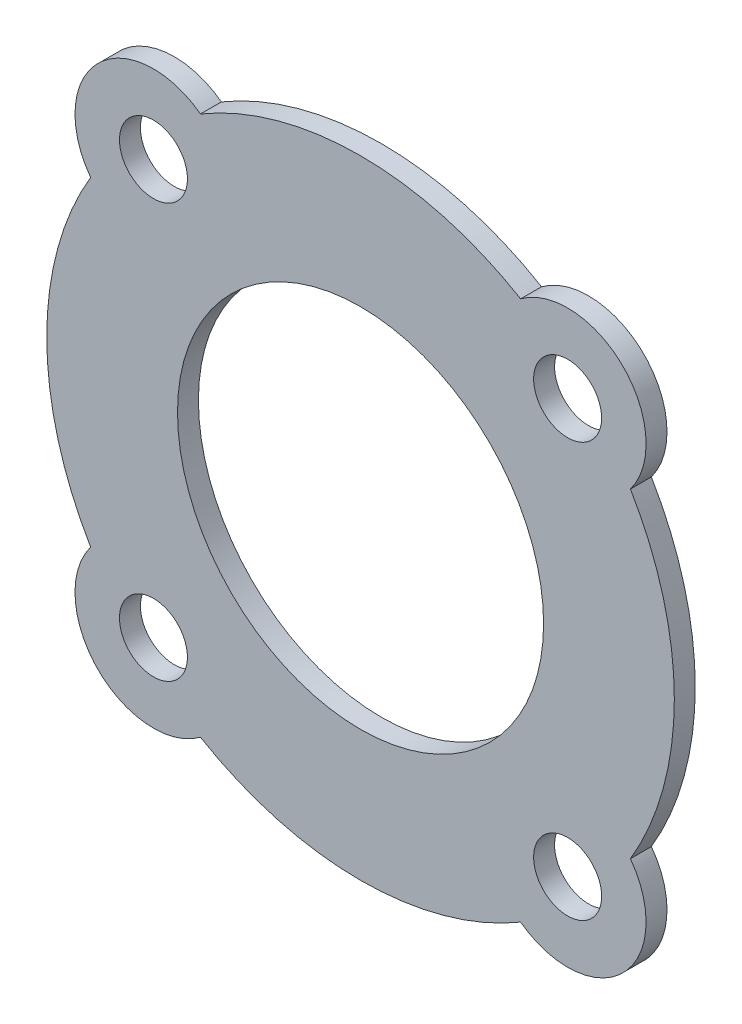
SolidWorks part; units mm, degrees
ref_plane "Front Plane" through (0, 0, 0) normal (0, 0, 1) x (1, 0, 0)
ref_plane "Top Plane" through (0, 0, 0) normal (0, 1, 0) x (1, 0, 0)
ref_plane "Right Plane" through (0, 0, 0) normal (1, 0, 0) x (0, 0, -1)
sketch "Sketch1" plane through (0, 0, 0) normal (0, 0, 1) x (1, 0, 0)
  line L0 (0, 0) -> (0, 56)
  line L1 (39.598, 39.598) -> (0, 0) construction
  circle A0 centre (0, 0) radius 35
  circle A1 centre (0, 0) radius 56 construction
  arc A2 (30.6082, 51.6056) -> (-30.6082, 51.6056) centre (0, 0) ccw
  circle A3 centre (39.598, 39.598) radius 6.5
  arc A4 (51.6056, 30.6082) -> (30.6082, 51.6056) centre (39.598, 39.598) ccw
  arc A5 (30.6082, -51.6056) -> (51.6056, -30.6082) centre (39.598, -39.598) ccw
  circle A6 centre (39.598, -39.598) radius 6.5
  arc A7 (-51.6056, -30.6082) -> (-30.6082, -51.6056) centre (-39.598, -39.598) ccw
  circle A8 centre (-39.598, -39.598) radius 6.5
  arc A9 (-30.6082, 51.6056) -> (-51.6056, 30.6082) centre (-39.598, 39.598) ccw
  circle A10 centre (-39.598, 39.598) radius 6.5
  arc A11 (-51.6056, 30.6082) -> (-51.6056, -30.6082) centre (0, 0) ccw
  arc A12 (-30.6082, -51.6056) -> (30.6082, -51.6056) centre (0, 0) ccw
  arc A13 (51.6056, -30.6082) -> (51.6056, 30.6082) centre (0, 0) ccw
  point P24 (0, 0)
  dimension "D1" = 70
  dimension "D2" = 112
  dimension "D3" = 120
  dimension "D4" = 13
  dimension "D5" = 30
  dimension "D6" = 45
  dimension "D7" = 4
extrude "Boss-Extrude1" add sketch "Sketch1" along normal mid plane 4
